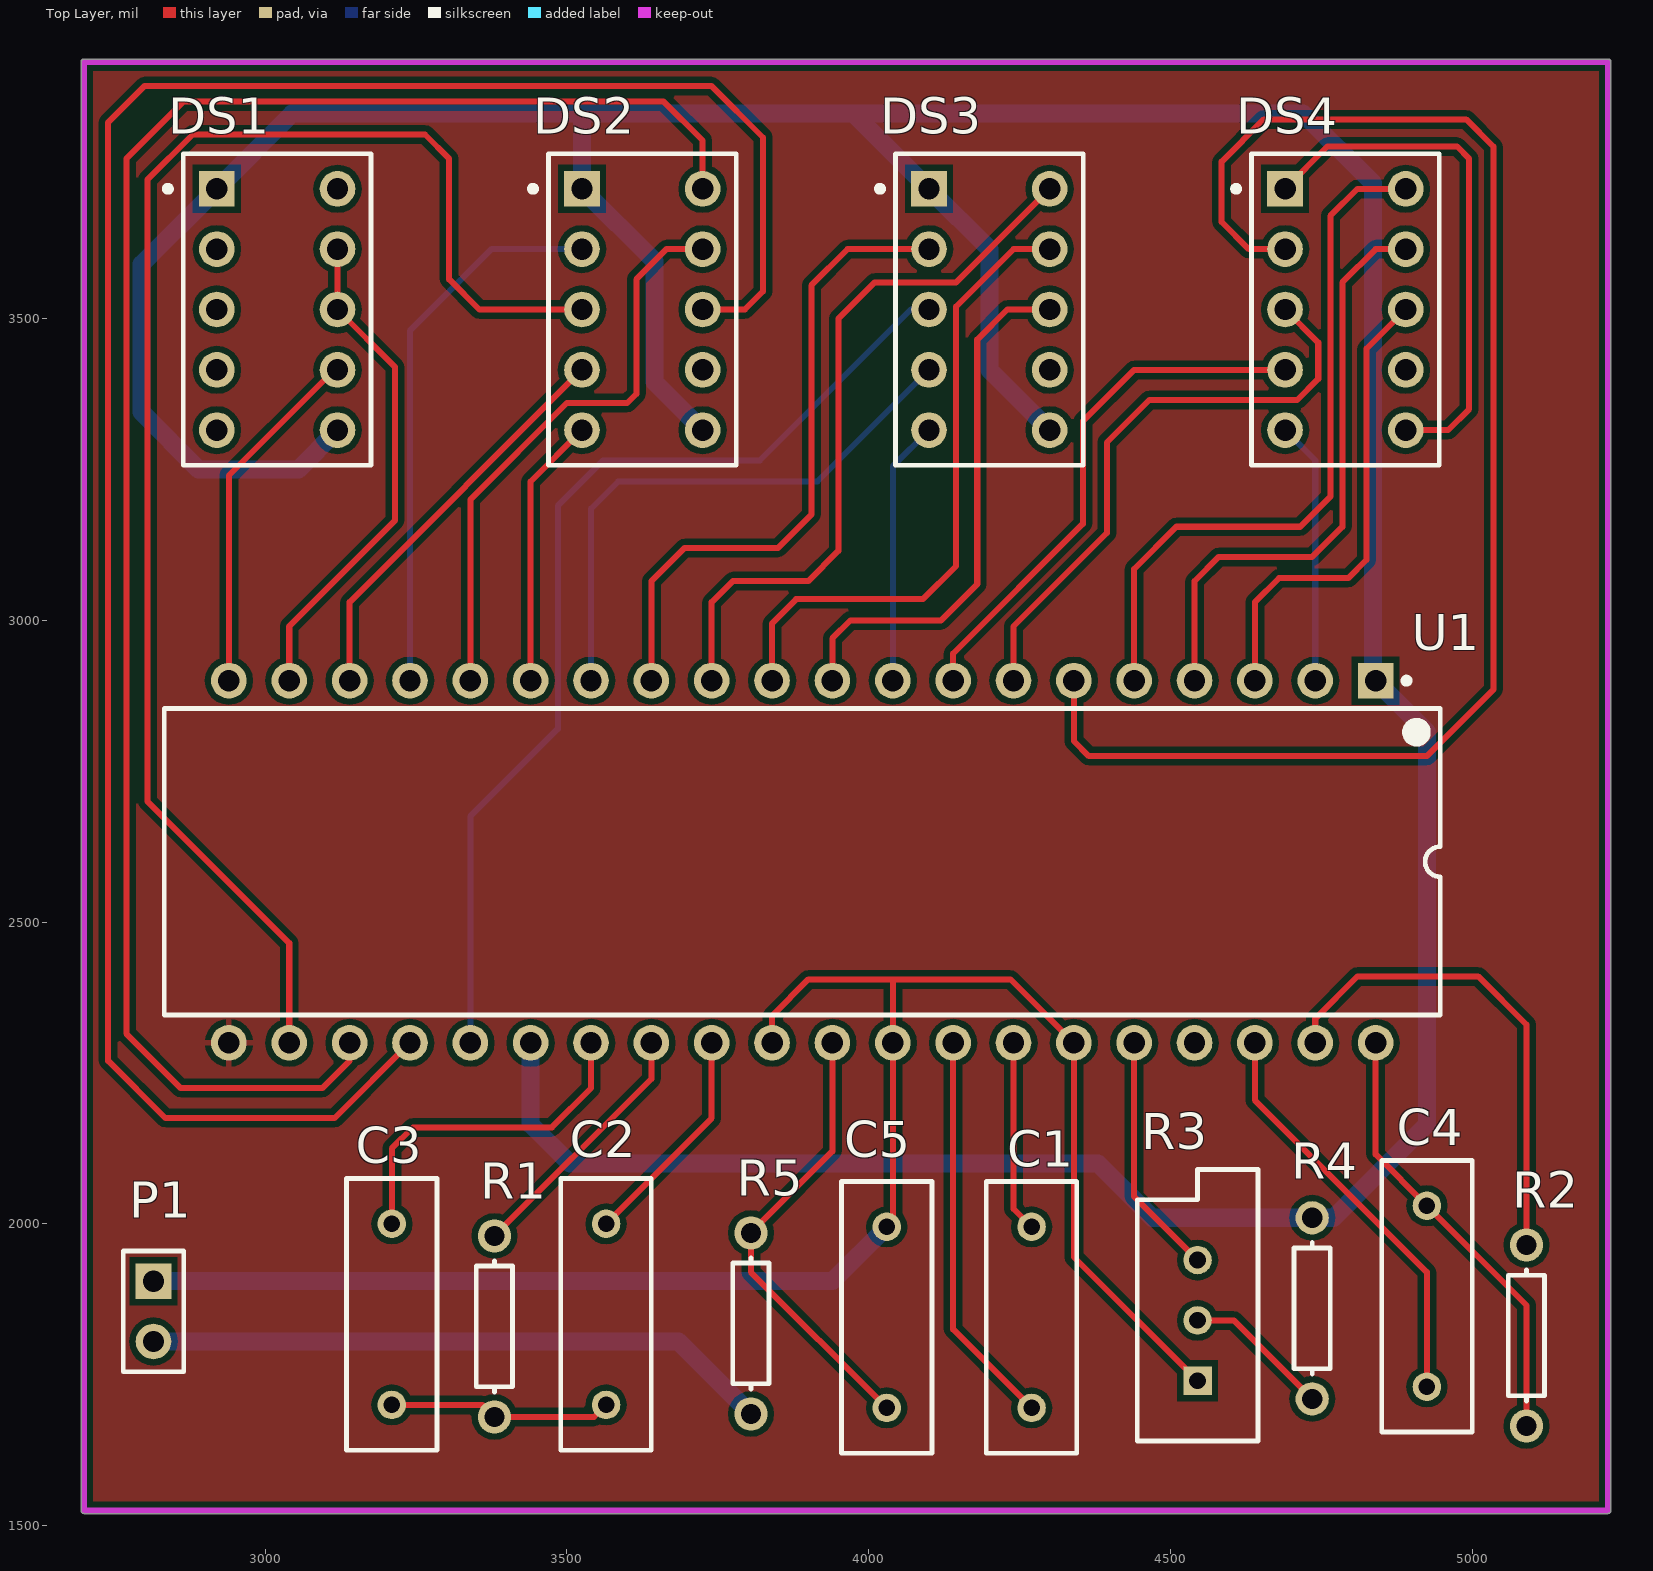
[diagram p0: Top Layer view]
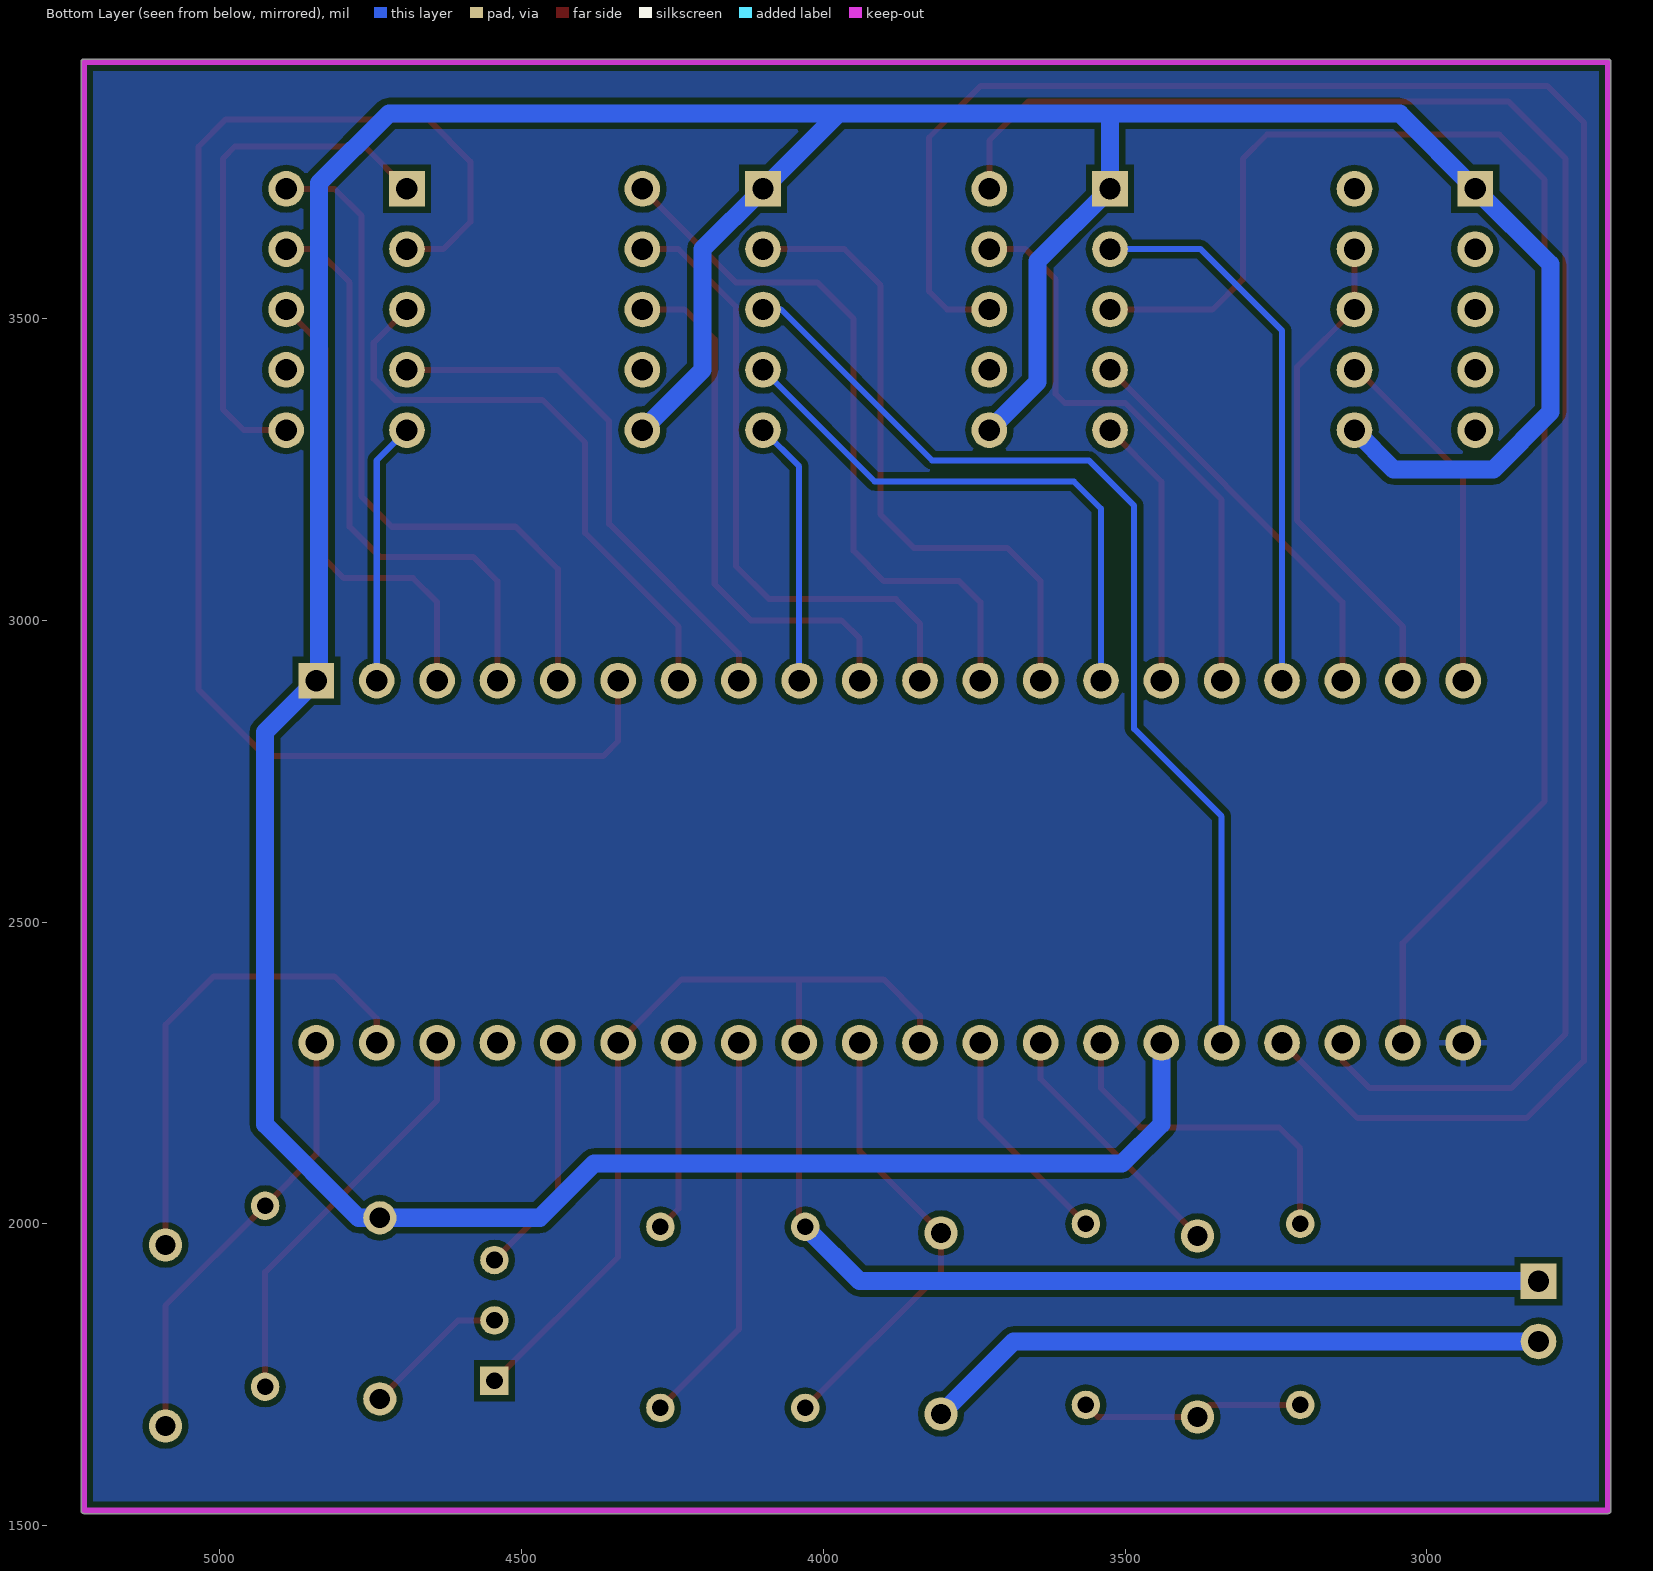
[diagram p1: Bottom Layer view, seen from below]
# Altium PCB MISC82817.PcbDoc
Units mil, origin at the board's own origin, x right, y up, seen from the top; angles counter-clockwise.
Board outline 2535.03 x 2410.03 mil, 2 copper layers (Top Layer, Bottom Layer); 16 components, 40 nets, 103 pads, 0 vias.

## Layer stack, top to bottom (the 12.6 mil dielectric is the usual default, probably not edited)
Top Solder: solder mask 0.4, Solder Resist, Dk 3.5
Top Layer: signal copper 1.4
Dielectric 1: dielectric 12.6, FR-4, Dk 4.8
Bottom Layer: signal copper 1.4
Bottom Solder: solder mask 0.4, Solder Resist, Dk 3.5

## Board outline
2694.99,1525 ccw(c2700,1525) 2700,1519.98 5225,1519.98 ccw(c5225,1525) 5230.02,1525 5230.02,3925 ccw(c5225,3925) 5225,3930.01 2700,3930.01 ccw(c2700,3925) 2694.99,3925

## Design rules (kind name [scope] priority, off if disabled: settings)
Clearance [All] p1: gap=10
MinimumSolderMaskSliver [All] p1: minsoldermaskwidth=0
PolygonConnect [All] p1: connectstyle=Relief reliefconductorwidth=10 reliefentries=4 polygonreliefangle="90 Angle" airgapwidth=10
RoutingVias [All] p1: holewidth=28 width=50 viastyle="Through Hole" minholewidth=28 minwidth=50 maxholewidth=28 maxwidth=50
SilkToSilkClearance [All] p1: silktosilkclearance=0
SilkToSolderMaskClearance [IsPad] p1: minsilkscreentomaskgap=0 clearancetoexposedcopper=TRUE
SolderMaskExpansion [All] p1: expansion=4
Width [All] p1: maxlimit=30 minlimit=10 preferedwidth=10
27 further rules are at their usual default settings.

## Components (designator, comment, footprint, x,y, rotation, side; value= is the part's Value field where it differs from the comment)
C1 "0.1UF" RAD-0.3 4270,1845 r270 top
C2 "0.47UF" RAD-0.3 3565,1850 r270 top
C3 "0.22UF" RAD-0.3 3210,1850 r270 top
C4 "100PF" RAD-0.3 4925,1880 r90 top
C5 "0.02UF" RAD-0.3 4030,1845 r270 top
DS1 "Dpy Green-CA" A 3020,3515 r0 top
DS2 "Dpy Green-CA" A 3625,3515 r0 top
DS3 "Dpy Green-CA" A 4200,3515 r0 top
DS4 "Dpy Green-CA" A 4790,3515 r0 top
P1 "+/-200MV input" HDR1X2 2815,1905 r270 top
R1 "1M" AXIAL-0.3 3380,1830 r90 top
R2 "100K" AXIAL-0.3 5090,1815 r90 top
R3 "24K" VR5 4545,1840 r90 top
R4 "24K" AXIAL-0.3 4735,1860 r270 top
R5 "1M" AXIAL-0.3 3805,1835 r90 top
U1 "ICL7107CJL" JL40A 3890,2600 r270 top

## Footprints (in the part's own frame and the unit in brackets; to place one, negate y for a bottom-side part, rotate by r counter-clockwise, add the part's x,y. Pads: shape width x height; smd on the part's side, far side on the other; paste and mask are expansions set on the pad)
A [mm] "LED, 7-Segment Display, 7.62 mm, RHD; 10 Leads; Row Space 5.08 mm; Pitch 2.54 mm"
  rect 1.5x1.5 hole 0.9: 1(-2.54,5.08)
  round 1.5 hole 0.9: 2(-2.54,2.54) 3(-2.54,0) 4(-2.54,-2.54) 5(-2.54,-5.08) 6(2.54,-5.08) 7(2.54,-2.54) 8(2.54,0) 9(2.54,2.54) 10(2.54,5.08)
  silkscreen extent -4.72,-6.55 3.95,6.55, body extent -3.95,-6.55 3.95,6.55, height 6.34
AXIAL-0.3 [mm] "Axial Device, Thru-Hole; 2 Leads; 0.3 in Pin Spacing"
  round 1.4 hole 0.85: 1(-3.81,0) 2(3.81,0)
  silkscreen extent -2.77,-0.76 2.77,0.76
HDR1X2 [mm] "Connector; Header; 2 Position"
  rect 1.5x1.5 hole 0.9: 1(0,0)
  round 1.5 hole 0.9: 2(2.54,0)
  silkscreen extent -1.27,-1.27 3.81,1.27
JL40A [mm] "DIP, 40-Leads, Row Spacing 15.24mm, Pitch 2.54mm, Body 52.28x14.35mm"
  rect 1.5x1.5 hole 0.9: 1(-7.62,24.13)
  round 1.5 hole 0.9: 2(-7.62,21.59) 3(-7.62,19.05) 4(-7.62,16.51) 5(-7.62,13.97) 6(-7.62,11.43) 7(-7.62,8.89) 8(-7.62,6.35) 9(-7.62,3.81) 10(-7.62,1.27) 11(-7.62,-1.27) 12(-7.62,-3.81) 13(-7.62,-6.35) 14(-7.62,-8.89) 15(-7.62,-11.43) 16(-7.62,-13.97) 17(-7.62,-16.51) 18(-7.62,-19.05) 19(-7.62,-21.59) 20(-7.62,-24.13) 21(7.62,-24.13) 22(7.62,-21.59) 23(7.62,-19.05) 24(7.62,-16.51) 25(7.62,-13.97) 26(7.62,-11.43) 27(7.62,-8.89) 28(7.62,-6.35) 29(7.62,-3.81) 30(7.62,-1.27) 31(7.62,1.27) 32(7.62,3.81) 33(7.62,6.35) 34(7.62,8.89) 35(7.62,11.43) 36(7.62,13.97) 37(7.62,16.51) 38(7.62,19.05) 39(7.62,21.59) 40(7.62,24.13)
  silkscreen extent -7.74,-26.85 6.45,26.85, body extent -7.3,-26.85 7.3,26.85, height 5.72
RAD-0.3 [mm] "Radial Cap, Thru-Hole; 2 Leads; 0.3 in Pin Spacing"
  round 1.2 hole 0.7: 1(-3.81,0) 2(3.81,0)
  silkscreen extent -5.71,-1.91 5.71,1.91
VR5 [mm] "Thru-Hole; 3 Leads"
  rect 1.2x1.2 hole 0.7: 1(-2.54,0)
  round 1.2 hole 0.7: 2(0,0) 3(2.54,0)
  silkscreen extent -5.08,-2.54 6.35,2.54

## Part data
C1 C2 C3 C4 C5: library part Cap, "Capacitor"
DS1 DS2 DS3 DS4: "7.62 mm Black Surface Green 7-Segment Display: CA, RH DP"
P1: library part "Header 2", "Header, 2-Pin"
R1 R2 R4 R5: library part Res1, "Resistor"
R3: library part RPot, "Potentiometer"
U1: "3?Digit A/D Converter"

## Nets (pads, with @x,y where several pads share a name; then routed paths per layer and width w, separated by ;. In a path a pad name is that pad's centre, name@x,y a point inside that pad or via, vN(x,y) a via of type N, cw(c..) or ccw(c..) an arc to the next point about the centre after c; other vN are vias at no path point)
+5V: DS1.1 DS1.6 DS2.1 DS2.6 DS3.1 DS3.6 R4.1 U1.1 U1.26 | length 7440.6
  Bottom Layer w30: DS1.6 3055,3250 2890,3250 2795,3345 2795,3590 DS1.1 3045,3840 3525,3840 ; U1.26 3440,2165 3505,2100 4380,2100 4470,2010 R4.1 4770,2010 4925,2165 4925,2815 U1.1 4835.47,2904.53 4835.47,3724.53 4720,3840 3975,3840 ; DS2.6 3645,3395 3645,3595 DS2.1 3525,3840 ; DS3.6 4200,3415 4200,3615 DS3.1 3975,3840 ; 3525,3840 3975,3840
A1: DS4.10 U1.5 | length 1168.3
  Top Layer w10: U1.5 4440,3085 4510,3155 4715,3155 4765,3205 4765,3670 4810,3715 DS4.10
A2: DS3.10 U1.12 | length 1199.3
  Top Layer w10: U1.12 3740,3030 3775,3065 3900,3065 3950,3115 3950,3500 4010,3560 4145,3560 DS3.10
A3: DS2.10 U1.23 | length 3007.2
  Top Layer w10: U1.23 3140,2270 3095,2225 2860,2225 2770,2315 2770,3765 2865,3860 3660,3860 3725,3795 DS2.10
AB4: DS1.8 DS1.9 U1.19 | length 826.8
  Top Layer w10: U1.19 3040,2990 3215,3165 3215,3420 DS1.8 DS1.9
B1: DS4.9 U1.4 | length 980.1
  Top Layer w10: U1.4 4540,3065 4580,3105 4735,3105 4785,3155 4785,3560 4840,3615 DS4.9
B2: DS3.9 U1.11 | length 1063.7
  Top Layer w10: U1.11 3840,2995 3880,3035 4090,3035 4145,3090 4145,3520 4240,3615 DS3.9
B3: DS2.9 U1.16 | length 968.2
  Top Layer w10: U1.16 3340,3200 3500,3360 3600,3360 3615,3375 3615,3565 3665,3615 DS2.9
C1: DS4.8 U1.3 | length 785.9
  Top Layer w10: U1.3 4640,3030 4680,3070 4795,3070 4825,3100 4825,3450 DS4.8
C2: DS3.8 U1.10 | length 893
  Top Layer w10: U1.10 3940,2970 3970,3000 4120,3000 4180,3060 4180,3465 4230,3515 DS3.8
C3: DS2.8 U1.24 | length 3658.6
  Top Layer w10: U1.24 3115,2175 2835,2175 2740,2270 2740,3825 2800,3885 3740,3885 3825,3800 3825,3545 3795,3515 DS2.8
D1: DS4.5 U1.2 | length 435.7
  Bottom Layer w10: DS4.5 4740,3265 U1.2
D2: DS3.5 U1.9 | length 439.9
  Bottom Layer w10: U1.9 4040,3255 DS3.5
D3: DS2.5 U1.15 | length 450.2
  Top Layer w10: U1.15 3440,3230 DS2.5
E1: DS4.4 U1.8 | length 889.3
  Top Layer w10: U1.8 4140,2945 4355,3160 4355,3330 4440,3415 DS4.4
E2: DS3.4 U1.14 | length 940.3
  Bottom Layer w10: U1.14 3540,3185 3585,3230 3915,3230 DS3.4
E3: DS2.4 U1.18 | length 674.5
  Top Layer w10: U1.18 3140,3030 DS2.4
F1: DS4.2 U1.6 | length 2472.2
  Top Layer w10: U1.6 4340,2800 4365,2775 4925,2775 5035,2885 5035,3785 4990,3830 4655,3830 4585,3760 4585,3660 4630,3615 DS4.2
F2: DS3.2 U1.13 | length 1075.4
  Top Layer w10: U1.13 3640,3065 3695,3120 3850,3120 3905,3175 3905,3555 3965,3615 DS3.2
F3: DS2.2 U1.17 | length 920.9
  Bottom Layer w10: U1.17 3240,3480 3375,3615 DS2.2
G1: DS4.3 U1.7 | length 990.5
  Top Layer w10: U1.7 4240,2990 4395,3145 4395,3295 4465,3365 4710,3365 4745,3400 4745,3460 DS4.3
G2: DS3.3 U1.25 | length 1699.7
  Bottom Layer w10: U1.25 3340,2675 3485,2820 3485,3190 3560,3265 3820,3265 4070,3515 DS3.3
G3: DS2.3 U1.22 | length 2515.7
  Top Layer w10: U1.22 3040,2465 2805,2700 2805,3730 2880,3805 3265,3805 3305,3765 3305,3565 3355,3515 DS2.3
GND: U1.21
NetC1_1: C1.1 U1.34 | length 317.4
  Top Layer w10: U1.34 4240,2025 C1.1
NetC1_2: C1.2 U1.33 | length 658.8
  Top Layer w10: U1.33 4140,1825 C1.2
NetC2_1: C2.1 U1.29 | length 372.5
  Top Layer w10: C2.1 3740,2175 U1.29
NetC2_2: C2.2 C3.2 R1.1 | length 371.6
  Top Layer w10: C3.2 3360,1700 R1.1 3545,1680 C2.2
NetC3_1: C3.1 U1.27 | length 571.4
  Top Layer w10: C3.1 3210,2125 3245,2160 3475,2160 3540,2225 U1.27
NetC4_1: C4.1 U1.38 | length 688.1
  Top Layer w10: U1.38 4640,2205 4925,1920 C4.1
NetC4_2: C4.2 R2.1 U1.40 | length 738.6
  Top Layer w10: U1.40 4840,2115 C4.2 5090,1865 R2.1
NetC5_1: C5.1 P1.1 R3.1 U1.30 U1.32 U1.35 | length 2924.7
  Top Layer w10: U1.30 3840,2345 3900,2405 4040,2405 ; C5.1 4040,2005 U1.32 4040,2405 ; R3.1 4340,1945 U1.35 4235,2405 4040,2405
  Bottom Layer w30: P1.1 3940,1905 C5.1
NetC5_2: C5.2 R5.2 U1.31 | length 754.1
  Top Layer w10: U1.31 3940,2120 R5.2 3805,1920 C5.2
NetDS4_1: DS4.1 DS4.6 | length 876.8
  Top Layer w10: DS4.1 4760,3785 4975,3785 4995,3765 4995,3350 4960,3315 DS4.6
NetP1_2: P1.2 R5.1 | length 1039.7
  Bottom Layer w30: P1.2 3685,1805 R5.1
NetR1_2: R1.2 U1.28 | length 427.7
  Top Layer w10: R1.2 3640,2240 U1.28
NetR2_2: R2.2 U1.39 | length 817.1
  Top Layer w10: U1.39 4740,2340 4810,2410 5010,2410 5090,2330 R2.2
NetR3_2: R3.2 R4.2 | length 243.8
  Top Layer w10: R3.2 4605,1840 R4.2
NetR3_3: R3.3 U1.36 | length 403.5
  Top Layer w10: U1.36 4440,2045 R3.3
POL: DS1.7 U1.20 | length 592.5
  Top Layer w10: U1.20 2940,3240 3115,3415 DS1.7
pads on no net: DS1.2 DS1.3 DS1.4 DS1.5 DS1.10 DS2.7 DS3.7 DS4.7 U1.37

## Polygon pours and split planes (outlines as drawn)
GND on Bottom Layer "D" (solid, remove dead copper, pour order 0): 2460,4150 2485,4125 5440,4125 5440,1260 5300,1120 5160,1260 2375,1260
GND on Top Layer "D" (solid, remove dead copper, pour order 2): 2345,4125 5450,4125 5525,4200 5390,4065 5390,810 2660,810 2290,1180

## Keep-outs
Keep-Out Layer:
  lines w10: 2825,3925 5130,3925 5225,3925 5225,1525 2700,1525 2700,3925 2845,3925